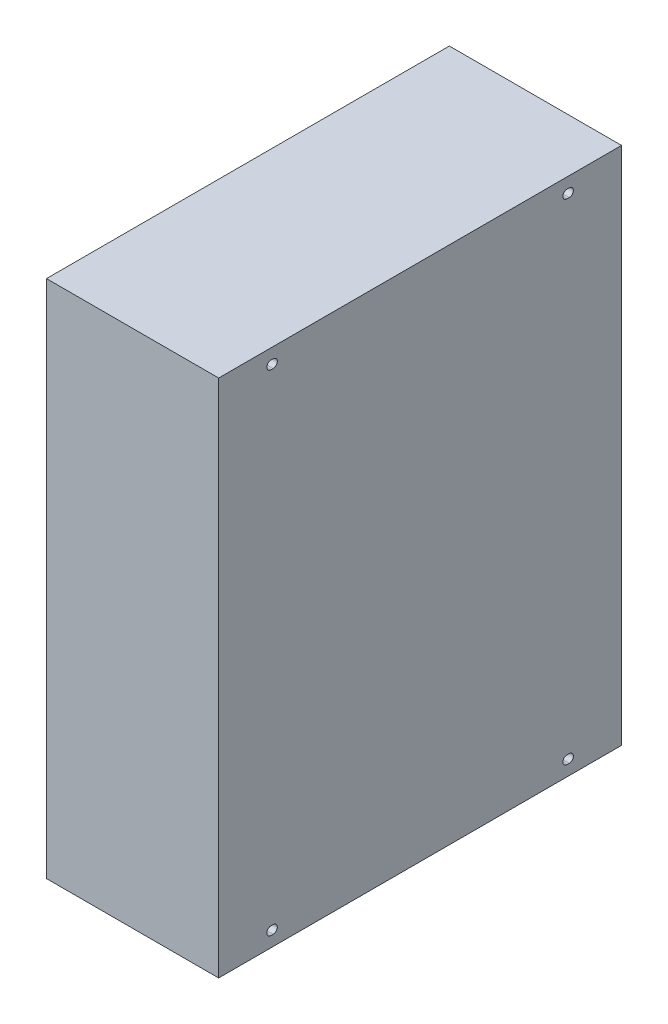
SolidWorks part; units mm, degrees
material "SPCC冷轧板喷塑"
ref_plane "前视基准面" through (0, 0, 0) normal (0, 0, 1) x (1, 0, 0)
ref_plane "上视基准面" through (0, 0, 0) normal (0, 1, 0) x (1, 0, 0)
ref_plane "右视基准面" through (0, 0, 0) normal (1, 0, 0) x (0, 0, -1)
other "Configuration Table"
sketch "草图1" plane through (0, 0, 0) normal (1, 0, 0) x (0, 0, -1)
  line L1 (287.8, -371.2) -> (-287.8, -371.2)
  line L2 (287.8, -371.2) -> (287.8, 371.2)
  line L3 (287.8, 371.2) -> (-287.8, 371.2)
  line L4 (-287.8, -371.2) -> (-287.8, 371.2)
  line L5 (287.8, -371.2) -> (-287.8, 371.2) construction
  line L6 (287.8, 371.2) -> (-287.8, -371.2) construction
  point P0 (0, 0)
  dimension "D1" = 742.4
  dimension "D2" = 575.6
extrude "凸台-拉伸1" add sketch "草图1" along normal mid plane 246
sketch "草图2" plane through (123, 0, 0) normal (1, 0, 0) x (0, 0, -1)
  line L0 (-213, 350) -> (-210, 350) construction
  line L3 (-213, 356) -> (-210, 356)
  line L4 (-213, 344) -> (-210, 344)
  line L5 (210, 350) -> (213, 350) construction
  line L6 (210, 356) -> (213, 356)
  line L7 (210, 344) -> (213, 344)
  line L8 (210, -350) -> (213, -350) construction
  line L9 (210, -344) -> (213, -344)
  line L10 (210, -356) -> (213, -356)
  line L11 (-213, -350) -> (-210, -350) construction
  line L12 (-213, -344) -> (-210, -344)
  line L13 (-213, -356) -> (-210, -356)
  line L14 (-213, 350) -> (210, 350) construction
  line L15 (-213, 350) -> (-213, -350) construction
  arc A2 (-213, 356) -> (-213, 344) centre (-213, 350) ccw
  arc A3 (-210, 344) -> (-210, 356) centre (-210, 350) ccw
  arc A4 (210, 356) -> (210, 344) centre (210, 350) ccw
  arc A5 (213, 344) -> (213, 356) centre (213, 350) ccw
  arc A6 (210, -344) -> (210, -356) centre (210, -350) ccw
  arc A7 (213, -356) -> (213, -344) centre (213, -350) ccw
  arc A8 (-213, -344) -> (-213, -356) centre (-213, -350) ccw
  arc A9 (-210, -356) -> (-210, -344) centre (-210, -350) ccw
  point P2 (-211.5, 350)
  point P12 (211.5, 350)
  point P19 (211.5, -350)
  point P26 (-211.5, -350)
  dimension "D2" = 15
  dimension "D1" = 12
  dimension "D3" = 211.5
  dimension "D4" = 350
  dimension "D7" = 423
  dimension "D8" = 700
  dimension "D5" = 2
  dimension "D6" = 2
extrude "切除-拉伸1" cut sketch "草图2" against normal through all
